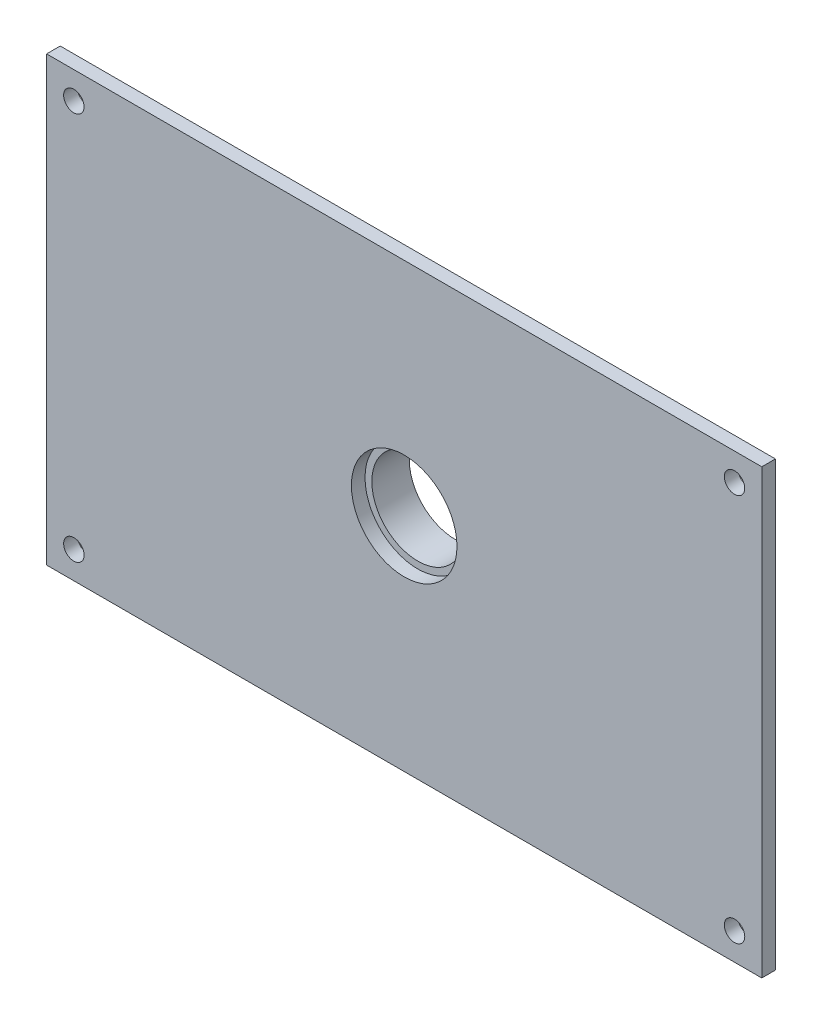
from build123d import *

# Parameters (mm, degrees)
SKETCH1_W           = 210
SKETCH1_H           = 130
SKETCH1_R           = 3
BOSS_EXTRUDE1_DEPTH = 4
SKETCH2_W           = 48
SKETCH2_H           = 48
BOSS_EXTRUDE2_DEPTH = 11
SKETCH3_R           = 13.5
CUT_EXTRUDE1_DEPTH  = 11
SKETCH4_R           = 15.5
CUT_EXTRUDE2_DEPTH  = 11
SCALE_1_SCALE       = 1.875


with BuildPart() as part:
    # Sketch1 → Boss-Extrude1 (new body)
    with BuildSketch(Plane.XY):
        Rectangle(SKETCH1_W, SKETCH1_H)
        with Locations((97, 57)):
            Circle(SKETCH1_R, mode=Mode.SUBTRACT)
        with Locations((-97, 57)):
            Circle(SKETCH1_R, mode=Mode.SUBTRACT)
        with Locations((-97, -57)):
            Circle(SKETCH1_R, mode=Mode.SUBTRACT)
        with Locations((97, -57)):
            Circle(SKETCH1_R, mode=Mode.SUBTRACT)
    extrude(amount=BOSS_EXTRUDE1_DEPTH)

    # Sketch2 → Boss-Extrude2 (add)
    with BuildSketch(Plane(origin=(0, 0, 0), x_dir=(-1, 0, 0), z_dir=(0, 0, -1))):
        Rectangle(SKETCH2_W, SKETCH2_H)
    extrude(amount=BOSS_EXTRUDE2_DEPTH)

    # Sketch3 → Cut-Extrude1 (cut)
    with BuildSketch(Plane(origin=(0, 0, -11), x_dir=(-1, 0, 0), z_dir=(0, 0, -1))):
        Circle(SKETCH3_R)
    extrude(amount=-CUT_EXTRUDE1_DEPTH, mode=Mode.SUBTRACT)

    # Sketch4 → Cut-Extrude2 (cut)
    with BuildSketch(Plane(origin=(0, 0, 0), x_dir=(-1, 0, 0), z_dir=(0, 0, -1))):
        Circle(SKETCH4_R)
    extrude(amount=-CUT_EXTRUDE2_DEPTH, mode=Mode.SUBTRACT)


with BuildPart() as part_1:
    # Scale 1: scaled about (0, 0, 0.855180598)
    add(part.part.scale(SCALE_1_SCALE).moved(Location((0, 0, -0.748283023))))


solid = part_1.part
